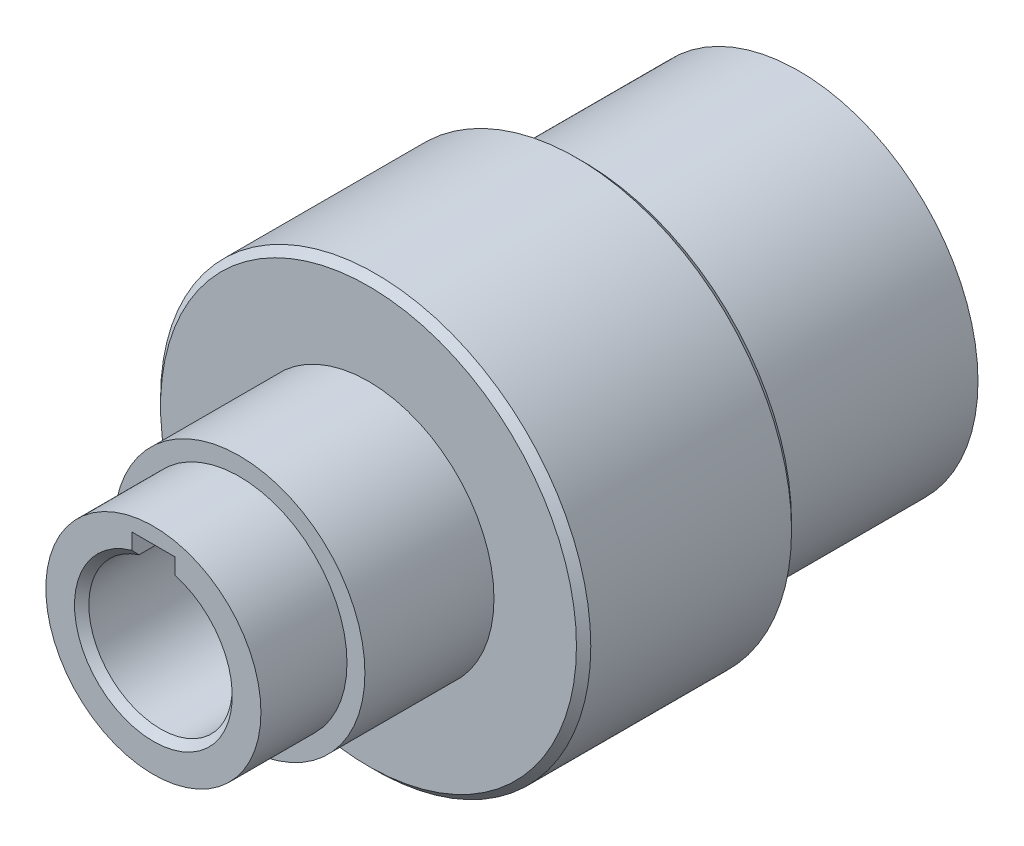
from build123d import *

# Parameters (mm, degrees)
SKETCH_1_R          = 25
EXTRUDE_1_DEPTH     = 30
SKETCH_2_R          = 30
EXTRUDE_2_DEPTH     = 40
SKETCH_4_R          = 10
CUT_EXTRUDE_1_DEPTH = 82.853527719
SKETCH_11_W         = 6
SKETCH_11_H         = 3.260607986
CUT_EXTRUDE_3_DEPTH = 82.853527719
SKETCH_12_R         = 15
CUT_EXTRUDE_4_DEPTH = 30
SKETCH_13_R         = 17.5
EXTRUDE_4_DEPTH     = 20
CUT_EXTRUDE_START   = -10
SKETCH_14_R         = 30
SKETCH_14_R_2       = 17.5
CUT_EXTRUDE_5_DEPTH = 10
CUT_EXTRUDE_START_2 = -12
SKETCH_15_R         = 17.5
SKETCH_15_R_2       = 15
CUT_EXTRUDE_6_DEPTH = 12
CHAMFER_2_SIZE      = 1


with BuildPart() as part:
    # 草图1 → 凸台-拉伸1 (new body)
    with BuildSketch(Plane.XY):
        Circle(SKETCH_1_R)
    extrude(amount=EXTRUDE_1_DEPTH)

    # 草图2 → 凸台-拉伸2 (add)
    with BuildSketch(Plane.XY.offset(30)):
        Circle(SKETCH_2_R)
    extrude(amount=EXTRUDE_2_DEPTH)

    # 草图4 → 切除-拉伸1 (cut, through all)
    with BuildSketch(Plane(origin=(0, 0, 0), x_dir=(-1, 0, 0), z_dir=(0, 0, -1))):
        Circle(SKETCH_4_R)
    extrude(amount=-CUT_EXTRUDE_1_DEPTH, mode=Mode.SUBTRACT)

    # 草图11 → 切除-拉伸3 (cut, through all)
    with BuildSketch(Plane.XY.offset(70)):
        with Locations((0, 11.169696007)):
            Rectangle(SKETCH_11_W, SKETCH_11_H)
    extrude(amount=-CUT_EXTRUDE_3_DEPTH, mode=Mode.SUBTRACT)

    # 草图12 → 切除-拉伸4 (cut)
    with BuildSketch(Plane(origin=(0, 0, 0), x_dir=(-1, 0, 0), z_dir=(0, 0, -1))):
        Circle(SKETCH_12_R)
    extrude(amount=-CUT_EXTRUDE_4_DEPTH, mode=Mode.SUBTRACT)

    # 草图13 → 凸台-拉伸4 (add)
    with BuildSketch(Plane.XY.offset(70)):
        Circle(SKETCH_13_R)
        with BuildLine():
            Line((3, 9.539392014), (3, 12.8))
            Line((3, 12.8), (-3, 12.8))
            Line((-3, 12.8), (-3, 9.539392014))
            ThreePointArc((-3, 9.539392014), (0, -10), (3, 9.539392014))
        make_face(mode=Mode.SUBTRACT)
    extrude(amount=EXTRUDE_4_DEPTH)

    # 草图14 → 切除-拉伸5 (cut)
    with BuildSketch(Plane.XY.offset(70).offset(CUT_EXTRUDE_START)):
        Circle(SKETCH_14_R)
        Circle(SKETCH_14_R_2, mode=Mode.SUBTRACT)
    extrude(amount=CUT_EXTRUDE_5_DEPTH, mode=Mode.SUBTRACT)

    # 草图15 → 切除-拉伸6 (cut)
    with BuildSketch(Plane.XY.offset(90).offset(CUT_EXTRUDE_START_2)):
        Circle(SKETCH_15_R)
        with Locations(Location((0, 0, 0), (0, 0, 180))):
            Circle(SKETCH_15_R_2, mode=Mode.SUBTRACT)
    extrude(amount=CUT_EXTRUDE_6_DEPTH, mode=Mode.SUBTRACT)

    # 倒角2
    chamfer_2_edges = [part.edges().sort_by_distance(p)[0] for p in [
        (15, 0, 0),
        (0, -10, 90),
        (-30, 0, 30),
        (-30, 0, 60),
    ]]
    chamfer(chamfer_2_edges, length=CHAMFER_2_SIZE)


solid = part.part
